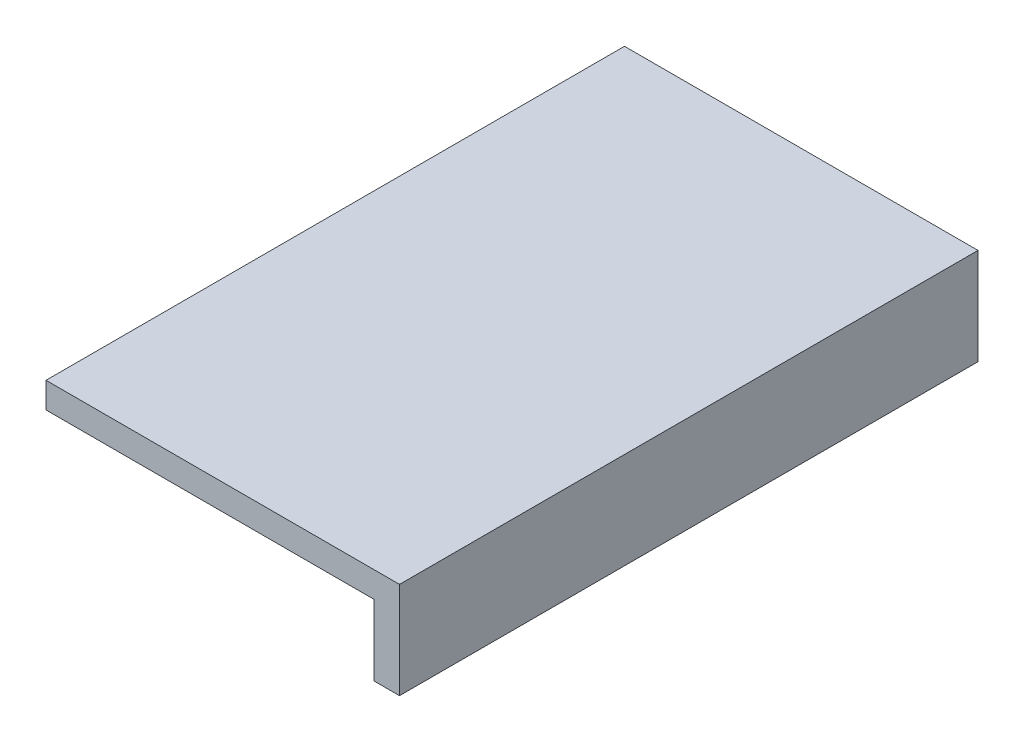
SolidWorks part; units mm, degrees
ref_plane "前视基准面" through (0, 0, 0) normal (0, 0, 1) x (1, 0, 0)
ref_plane "上视基准面" through (0, 0, 0) normal (0, 1, 0) x (1, 0, 0)
ref_plane "右视基准面" through (0, 0, 0) normal (1, 0, 0) x (0, 0, -1)
sketch "草图1" plane through (0, 0, 0) normal (0, 0, 1) x (1, 0, 0)
  line L0 (0, 0) -> (110, 0)
  line L1 (110, 0) -> (110, -30)
  line L2 (0, -8) -> (102, -8)
  line L3 (102, -8) -> (102, -30)
  line L4 (102, -30) -> (110, -30)
  line L5 (0, -8) -> (0, 0)
  dimension "D1" = 8
extrude "凸台-拉伸1" add sketch "草图1" along normal blind 180
